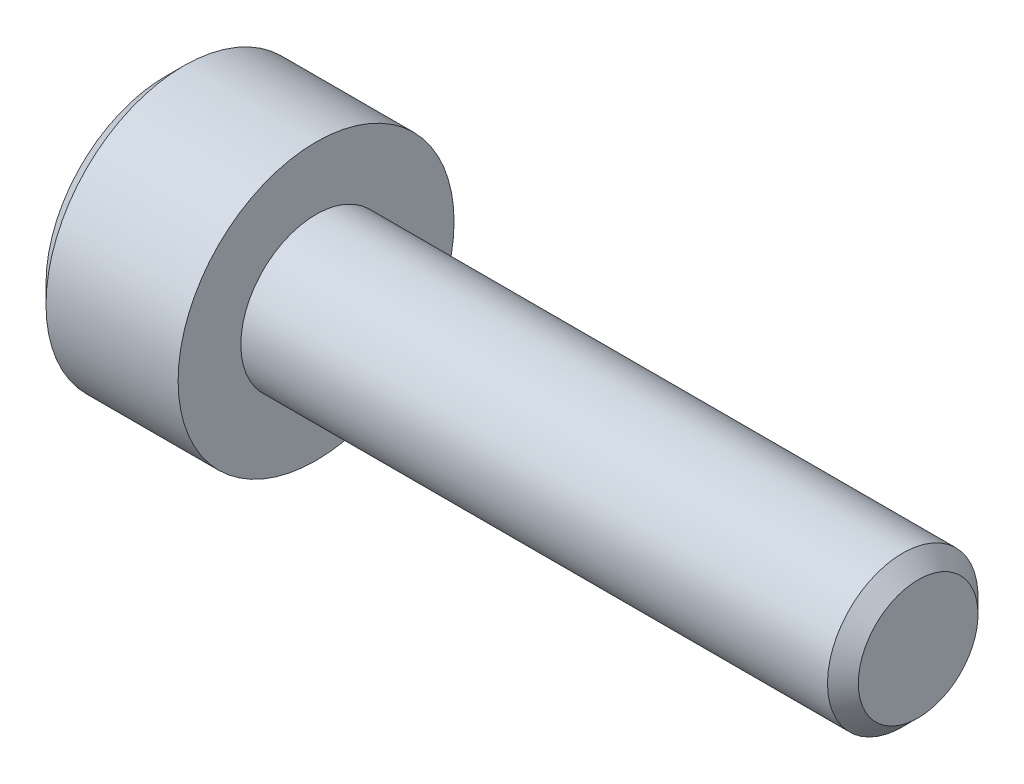
SolidWorks part; units mm, degrees
ref_plane "Front Plane" through (0, 0, 0) normal (0, 0, 1) x (1, 0, 0)
ref_plane "Top Plane" through (0, 0, 0) normal (0, 1, 0) x (1, 0, 0)
ref_plane "Right Plane" through (0, 0, 0) normal (1, 0, 0) x (0, 0, -1)
sketch "Sketch1" plane through (0, 0, 0) normal (0, 0, 1) x (1, 0, 0)
  line L0 (-3, 0) -> (-3, 2.3833)
  line L1 (-3, 2.3833) -> (-2.6333, 2.75)
  line L2 (-2.6333, 2.75) -> (0, 2.75)
  line L3 (0, 2.75) -> (0, 1.5)
  line L4 (0, 1.5) -> (11.6928, 1.5)
  line L5 (11.6928, 1.5) -> (12, 1.1928)
  line L6 (12, 1.1928) -> (12, 0)
  line L7 (12, 0) -> (-3, 0)
  line L8 (12, 0) -> (-3, 0) construction
revolve "Revolve1" add sketch "Sketch1" angle 360 about L8
cosmetic thread "Cosmetic Thread1" parameters "D1"=11.468, "D2"=2.3857
sketch "Sketch2" plane through (0, 0, 0) normal (0, 0, 1) x (1, 0, 0)
  line L0 (-3, 0) -> (-3, 1.25)
  line L1 (-3, 1.25) -> (-1.5, 1.25)
  line L2 (-1.5, 1.25) -> (-1.1651, 0)
  line L3 (-1.1651, 0) -> (-3, 0)
  line L4 (-1.1651, 0) -> (-3, 0) construction
revolve "Cut-Revolve1" cut sketch "Sketch2" angle 360 about L4
ref_plane "Plane1" through (-3, 0, 0) normal (1, 0, 0) x (0, 0, -1)
sketch "Sketch3" plane through (-3, 0, 0) normal (1, 0, 0) x (0, 0, -1)
  line L0 (-1.25, 0.7217) -> (-1.25, -0.7217)
  line L1 (-1.25, -0.7217) -> (0, -1.4434)
  line L2 (0, -1.4434) -> (1.25, -0.7217)
  line L3 (1.25, -0.7217) -> (1.25, 0.7217)
  line L4 (1.25, 0.7217) -> (0, 1.4434)
  line L5 (0, 1.4434) -> (-1.25, 0.7217)
extrude "Cut-Extrude1" cut sketch "Sketch3" along normal blind 1.5
